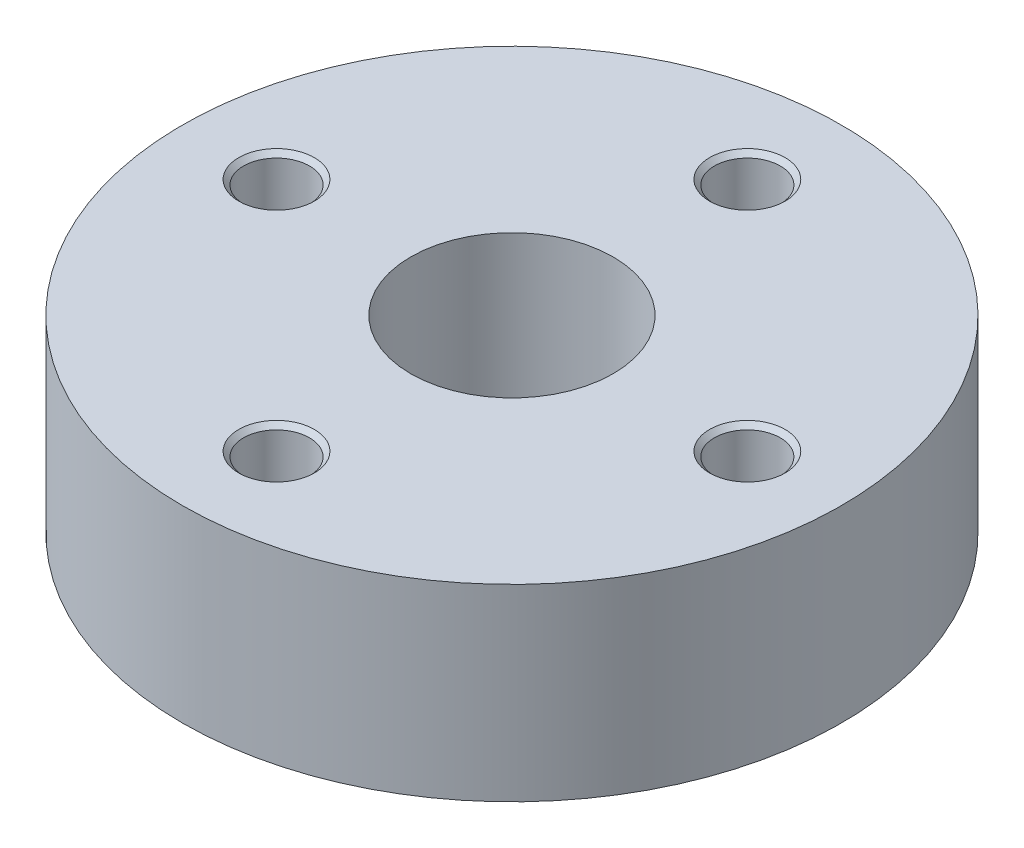
from build123d import *

# Parameters (mm, degrees)
SKETCH_1_R                    = 70
SKETCH_1_R_2                  = 21.5
EXTRUDE_1_DEPTH               = 40
HOLE_WIZARD_M16_1_D           = 14
HOLE_WIZARD_M16_1_DEPTH       = 27.793975667
HOLE_WIZARD_M16_1_CSINK_D     = 16.05
HOLE_WIZARD_M16_1_CSINK_ANGLE = 90
HOLE_WIZARD_M16_1_TIP         = 4.206024333
HOLE_WIZARD_M16_3_D           = 14
HOLE_WIZARD_M16_3_DEPTH       = 27.793975667
HOLE_WIZARD_M16_3_CSINK_D     = 16.05
HOLE_WIZARD_M16_3_CSINK_ANGLE = 90
HOLE_WIZARD_M16_3_TIP         = 4.206024333


with BuildPart() as part:
    # 草图1 → 凸台-拉伸1 (new body)
    with BuildSketch(Plane(origin=(0, 0, 0), x_dir=(1, 0, 0), z_dir=(0, 1, 0))):
        with Locations(Location((0, 0, 0), (0, 0, 270))):
            Circle(SKETCH_1_R)
        with Locations(Location((0, 0, 0), (0, 0, 270))):
            Circle(SKETCH_1_R_2, mode=Mode.SUBTRACT)
    extrude(amount=EXTRUDE_1_DEPTH)

    # M16 螺纹孔1
    with Locations(Plane(origin=(0, 40, 0), x_dir=(1, 0, 0), z_dir=(0, 1, 0))):
        with Locations((0, 50), (50, 0), (0, -50), (-50, 0)):
            CounterSinkHole(HOLE_WIZARD_M16_1_D / 2, HOLE_WIZARD_M16_1_CSINK_D / 2, depth=HOLE_WIZARD_M16_1_DEPTH, counter_sink_angle=HOLE_WIZARD_M16_1_CSINK_ANGLE)
            with Locations((0, 0, -(HOLE_WIZARD_M16_1_DEPTH + HOLE_WIZARD_M16_1_TIP / 2))):  # 118° drill point
                Cone(0, HOLE_WIZARD_M16_1_D / 2, HOLE_WIZARD_M16_1_TIP, mode=Mode.SUBTRACT)

    # M16 螺纹孔3
    with Locations(Plane(origin=(0, 0, 0), x_dir=(-1, 0, 0), z_dir=(0, -1, 0))):
        with Locations((-35.355339059, 35.355339059), (35.355339059, 35.355339059), (35.355339059, -35.355339059), (-35.355339059, -35.355339059)):
            CounterSinkHole(HOLE_WIZARD_M16_3_D / 2, HOLE_WIZARD_M16_3_CSINK_D / 2, depth=HOLE_WIZARD_M16_3_DEPTH, counter_sink_angle=HOLE_WIZARD_M16_3_CSINK_ANGLE)
            with Locations((0, 0, -(HOLE_WIZARD_M16_3_DEPTH + HOLE_WIZARD_M16_3_TIP / 2))):  # 118° drill point
                Cone(0, HOLE_WIZARD_M16_3_D / 2, HOLE_WIZARD_M16_3_TIP, mode=Mode.SUBTRACT)


solid = part.part
